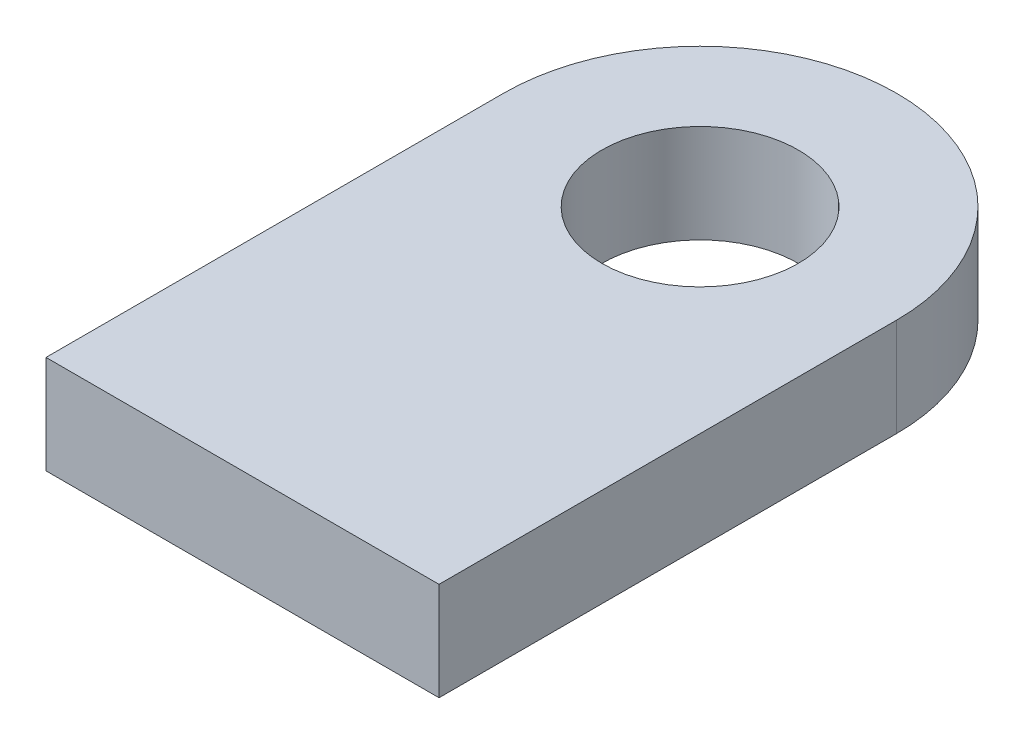
SolidWorks part; units mm, degrees
ref_plane "前视基准面" through (0, 0, 0) normal (0, 0, 1) x (1, 0, 0)
ref_plane "上视基准面" through (0, 0, 0) normal (0, 1, 0) x (1, 0, 0)
ref_plane "右视基准面" through (0, 0, 0) normal (1, 0, 0) x (0, 0, -1)
sketch "草图1" plane through (0, 0, 0) normal (0, 1, 0) x (1, 0, 0)
  line L1 (-20, -23.285) -> (20, -23.285)
  line L2 (-20, -23.285) -> (-20, 23.285)
  line L4 (20, -23.285) -> (20, 23.285)
  line L5 (-20, -23.285) -> (20, 23.285) construction
  line L6 (-20, 23.285) -> (20, -23.285) construction
  arc A1 (20, 23.285) -> (-20, 23.285) centre (0, 23.285) ccw
  circle A2 centre (0, 23.285) radius 10
  point P0 (0, 0)
  dimension "D3" = 20
  dimension "D5" = 20
  dimension "D2" = 40
  dimension "D4" = 46.57
extrude "凸台-拉伸1" add sketch "草图1" along normal mid plane 10
